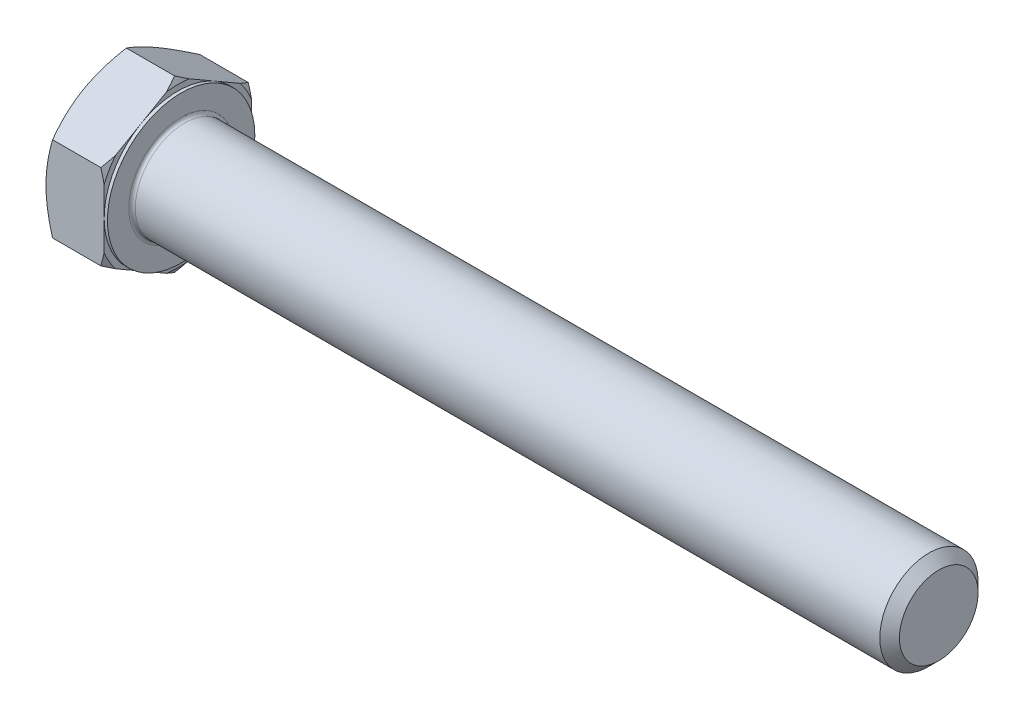
SolidWorks part; units mm, degrees
extrude "Base-Extrude" add sketch "Sketch1" along normal blind 15
sketch "Sketch1" plane through (0, 0, 0) normal (1, 0, 0) x (0, 0, -1)
  line L0 (18, 10.3923) -> (18, -10.3923)
  line L1 (-18, 10.3923) -> (-18, -10.3923)
  line L2 (18, -10.3923) -> (0, -20.7846)
  line L3 (0, -20.7846) -> (-18, -10.3923)
  line L4 (18, 10.3923) -> (0, 20.7846)
  line L5 (0, 20.7846) -> (-18, 10.3923)
revolve "Cut-Revolve1" cut sketch "Sketch3" angle 360 about L6
sketch "Sketch3" plane through (0, 0, 0) normal (0, 0, 1) x (1, 0, 0)
  line L0 (0, 18) -> (4.4944, 25.7846)
  line L1 (0, 20.7846) -> (0, 10.3923) construction
  line L2 (4.4944, 25.7846) -> (4.4944, 30.7846)
  line L3 (4.4944, 30.7846) -> (-10, 30.7846)
  line L4 (-10, 30.7846) -> (-10, 18)
  line L5 (-10, 18) -> (0, 18)
  line L6 (0, 0) -> (99.06, 0) construction
  line L7 (15, 20.7846) -> (0, 20.7846) construction
ref_plane "front" through (0, 0, 0) normal (0, 0, 1) x (1, 0, 0)
ref_plane "top" through (0, 0, 0) normal (0, 1, 0) x (1, 0, 0)
ref_plane "right" through (0, 0, 0) normal (1, 0, 0) x (0, 0, -1)
sketch "Sketch2" plane through (0, 0, 0) normal (0, 0, 1) x (1, 0, 0)
  line L0 (0, 10.3923) -> (0, -10.3923) construction
  line L1 (0, 0) -> (200, 0)
  line L2 (0, 0) -> (0, 12)
  line L3 (0, 12) -> (27.8072, 12)
  line L4 (200, 0) -> (200, 9.402)
  line L5 (15, 20.7846) -> (15, 10.3923) construction
  line L7 (0, 0) -> (96.52, 0) construction
  line L8 (200, -9.402) -> (27.8072, -12) construction
  line L9 (0, -12) -> (27.8072, -12) construction
  line L10 (18, 15.24) -> (18, -1.27) construction
  line L11 (140, 15.24) -> (140, -1.27) construction
  line L12 (15, 10.3923) -> (15, -10.3923) construction
  line L13 (27.8072, 12) -> (200, 12)
  line L14 (200, 12) -> (200, 9.402)
revolve "Boss-Revolve1" add sketch "Sketch2" angle 360 about L7
cosmetic thread "helix 1" parameters "Thread_length"=60, "Thread_minor"=18.804
sketch "Sketch5" plane through (0, 0, 0) normal (0, 0, 1) x (1, 0, 0)
  line L0 (15, 18) -> (10.5056, 25.7846)
  line L1 (15, 20.7846) -> (15, 10.3923) construction
  line L2 (10.5056, 25.7846) -> (10.5056, 30.7846)
  line L3 (10.5056, 30.7846) -> (20.5056, 30.7846)
  line L4 (20.5056, 30.7846) -> (20.5056, 18)
  line L5 (20.5056, 18) -> (15, 18)
  line L7 (15, 20.7846) -> (1.6077, 20.7846) construction
  line L8 (0, 0) -> (99.06, 0) construction
  line L9 (0, 0) -> (99.06, 0) construction
revolve "Cut-Revolve2" cut sketch "Sketch5" angle 360 about L8
sketch "Sketch4" plane through (0, 0, 0) normal (0, 0, 1) x (1, 0, 0)
  line L1 (15, 20.7846) -> (15, 10.3923) construction
  line L2 (15, 18) -> (14.2, 18)
  line L3 (15, 18) -> (15, 30.7846)
  line L4 (15, 30.7846) -> (14.2, 30.7846)
  line L5 (0, 0) -> (95.25, 0) construction
  line L6 (0, 0) -> (96.52, 0) construction
  line L7 (14.2, 18) -> (14.2, 30.7846)
  line L8 (13.3923, 20.7846) -> (1.6077, 20.7846) construction
revolve "Cut-Revolve3" cut sketch "Sketch4" angle 360 about L5
chamfer "Chamfer" distance 2.4 angle 45 1 edges at (200, 0, 12)
fillet "Fillet" radius 0.8 1 edges at (15, 0, -12)
sketch "Sketch6" plane through (0, 0, 0) normal (0, 0, 1) x (1, 0, 0)
  line L0 (140, -9.402) -> (138.5, -12)
  line L1 (140, -9.402) -> (141.5, -12)
  line L2 (141.5, -12) -> (141.5, -15)
  line L3 (-3.175, 0) -> (5.1513, 0) construction
  line L5 (141.5, -15) -> (138.5, -15)
  line L6 (138.5, -15) -> (138.5, -12)
revolve "Cut-Revolve4" [suppressed] cut sketch "Sketch6" angle 360 about L3
pattern_linear "LPattern1" [suppressed]
equation "\"D3@Sketch1\" = \"s@Sketch1\" / 2"
equation "\"D4@Sketch1\" = \"D3@Sketch1\""
equation "\"D5@Sketch1\" = \"D4@Sketch1\""
equation "\"Thread_minor@helix 1\" = \"Minor_dia@Sketch2\""
equation "\"D1@Sketch3\" = \"s@Sketch1\" / 2"
equation "\"D1@Sketch5\" = \"s@Sketch1\" / 2"
equation "\"Head_ch_ang@Sketch5\" = \"Head_ch_ang@Sketch3\""
equation "\"D1@Sketch4\" = \"s@Sketch1\""
equation "\"Thread_length@helix 1\" = ((sgn( (\"l@Sketch2\" - \"p@Sketch2\" ) - \"h@Sketch2\" )-1)*( (\"l@Sketch2\" - \"p@Sketch2\" ) - \"h@Sketch2\" ))/-2+ \"h@Sketch2\""
equation "\"Thread_minor@Sketch6\" = \"Minor_dia@Sketch2\""
equation "\"Diameter@Sketch6\" = \"m@Sketch2\""
equation "\"Overcut@Sketch6\" = \"m@Sketch2\" * 1.25"
equation "\"Start@Sketch6\" = \"k@Base-Extrude\" + \"l@Sketch2\" - \"Thread_length@helix 1\"  '---Non-countersunk---"
equation "\"Num_threads@LPattern1\" = int( \"Thread_length@helix 1\" / \"p@Sketch2\" + 0.999 )  + 1"
equation "\"Advance@LPattern1\" = \"Thread_length@helix 1\" /  (\"Num_threads@LPattern1\" - 1) 'relax it"
equation "\"Num_threads@LPattern1\" = \"Num_threads@LPattern1\" - sgn( \"Num_threads@LPattern1\" - 1) '---chamfered tips oxxx---"
equation "\"Minor_dia@Sketch2\" = \"m@Sketch2\"-\"p@Sketch2\" * 1.732"
equation "\"D1@Chamfer\" = \"p@Sketch2\"*0.8"
